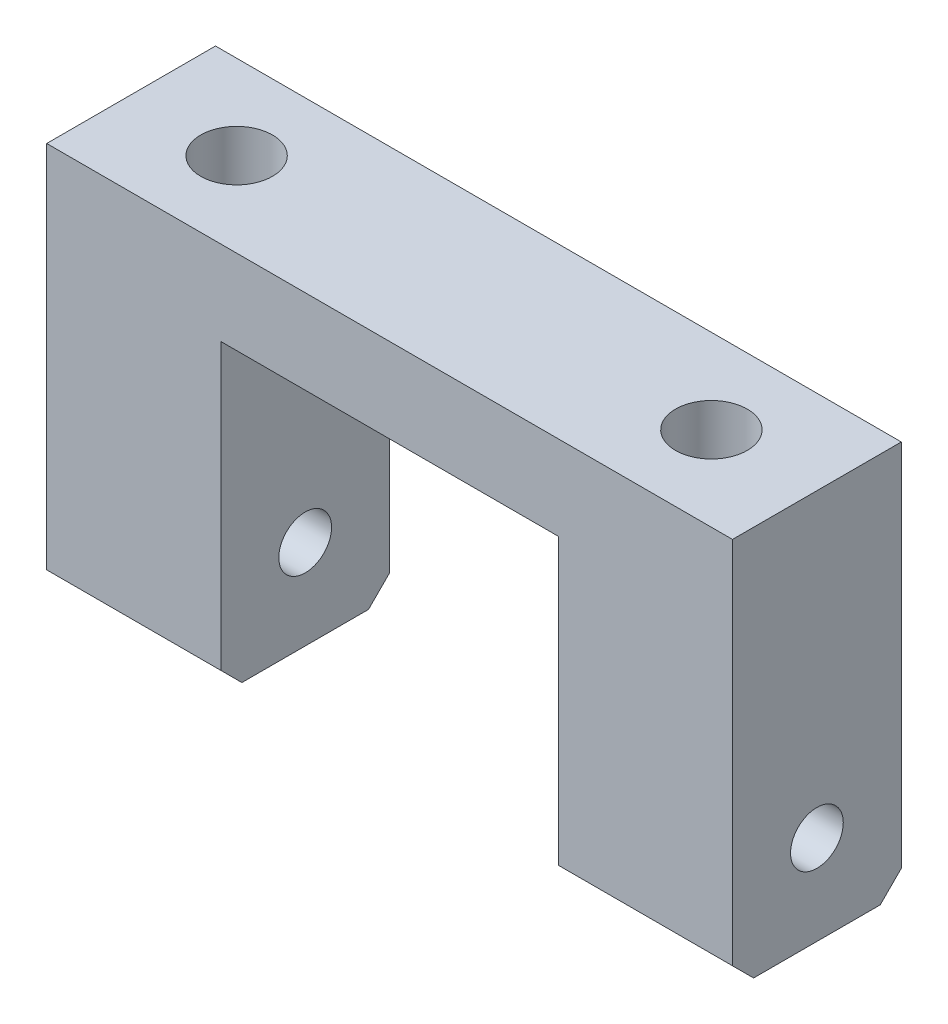
SolidWorks part; units mm, degrees
ref_plane "前视基准面" through (0, 0, 0) normal (0, 0, 1) x (1, 0, 0)
ref_plane "上视基准面" through (0, 0, 0) normal (0, 1, 0) x (1, 0, 0)
ref_plane "右视基准面" through (0, 0, 0) normal (1, 0, 0) x (0, 0, -1)
sketch "草图1" plane through (0, 0, 0) normal (0, 0, 1) x (1, 0, 0)
  line L0 (0, 18.5) -> (0, 0) construction
  line L1 (-32.5, 18.5) -> (32.5, 18.5)
  line L2 (-32.5, 18.5) -> (-32.5, -18.5)
  line L3 (-32.5, -18.5) -> (32.5, -18.5)
  line L4 (32.5, 18.5) -> (32.5, -18.5)
  line L5 (0, 0) -> (32.5, 0) construction
  dimension "D1" = 65
  dimension "D2" = 37
extrude "凸台-拉伸1" add sketch "草图1" along normal mid plane 16
sketch "草图3" plane through (0, 0, 8) normal (0, 0, 1) x (1, 0, 0)
  line L0 (-32.5, -18.5) -> (32.5, -18.5) construction
  line L1 (-16, -18.5) -> (16, -18.5)
  line L2 (-16, -18.5) -> (-16, 10.5)
  line L3 (-16, 10.5) -> (16, 10.5)
  line L4 (16, -18.5) -> (16, 10.5)
  line L5 (0, 29) -> (0, 0) construction
  line L6 (0, 0) -> (44.4811, 0) construction
  line L7 (32.5, 18.5) -> (-32.5, 18.5) construction
  dimension "D1" = 32
  dimension "D2" = 8
extrude "切除-拉伸1" cut sketch "草图3" against normal through all
hole_wizard "M6 螺纹孔1" positions "草图7" profile "草图6" tap size "M6" standard "ISO" end condition through all
sketch "草图7" plane through (32.5, 0, 0) normal (1, 0, 0) x (0, 0, -1)
  line L0 (0, 0) -> (0, -16.1416) construction
  line L4 (-8, -18.5) -> (8, -18.5) construction
  point P0 (0, -10)
  dimension "D1" = 8.5
sketch "草图6" plane through (32.5, -10, 0) normal (0, 1, 0) x (0, 0, -1)
  line L0 (0, 0) -> (0, 65)
  line L1 (0, 65) -> (2.5, 65)
  line L2 (2.5, 65) -> (2.5, 0)
  line L5 (2.5, 0) -> (0, 0)
  line L11 (0, -6.35) -> (0, 107.95) construction
  dimension "通孔螺纹孔钻头直径" = 5
  dimension "通孔螺纹孔钻头深度" = 65
cosmetic thread "孔螺蚊线4" parameters "D2"=6
hole_wizard "M8 螺纹孔1" positions "草图9" profile "草图8" tap size "M8" standard "Iso"
sketch "草图9" plane through (0, 23.5, 0) normal (0, 1, 0) x (1, 0, 0)
  line L0 (0, 13.8881) -> (0, 0) construction
  line L1 (0, 0) -> (44.4811, 0) construction
  point P0 (-32.5, 0)
  point P2 (32.5, 0)
  dimension "D1" = 65
sketch "草图8" plane through (-32.5, 23.5, 0) normal (1, 0, 0) x (0, 0, 1)
  line L0 (0, 0) -> (0, 21.7929)
  line L1 (0, 21.7929) -> (3.4, 19.75)
  line L2 (3.4, 19.75) -> (3.4, 0)
  line L5 (3.4, 0) -> (0, 0)
  line L10 (0, 21.7929) -> (-3.4, 19.75) construction
  line L11 (0, -6.35) -> (0, 107.95) construction
  dimension "螺纹孔钻头直径" = 6.8
  dimension "螺纹孔钻头深度" = 19.75
  dimension "导头角度" = 118
cosmetic thread "孔螺蚊线2" [suppressed] parameters "D1"=16, "D2"=8
cosmetic thread "孔螺蚊线3" [suppressed] parameters "D1"=16, "D2"=8
hole_wizard "M8 螺纹孔2" positions "草图11" profile "草图10" tap size "M8" standard "GB"
sketch "草图11" plane through (0, 18.5, 0) normal (0, 1, 0) x (1, 0, 0)
  line L0 (-32.5, 0) -> (32.5, 0) construction
  line L1 (-32.5, -8) -> (-32.5, 8) construction
  line L2 (32.5, -8) -> (32.5, 8) construction
  point P0 (-22.5, 0)
  point P2 (22.5, 0)
  dimension "D1" = 10
  dimension "D2" = 10
sketch "草图10" plane through (-22.5, 18.5, 0) normal (1, 0, 0) x (0, 0, 1)
  line L0 (0, 0) -> (0, 24.2929)
  line L1 (0, 24.2929) -> (3.4, 22.25)
  line L2 (3.4, 22.25) -> (3.4, 0)
  line L5 (3.4, 0) -> (0, 0)
  line L10 (0, 24.2929) -> (-3.4, 22.25) construction
  line L11 (0, -6.35) -> (0, 107.95) construction
  dimension "螺纹孔钻头直径" = 6.8
  dimension "螺纹孔钻头深度" = 22.25
  dimension "导头角度" = 118
cosmetic thread "孔螺蚊线5" parameters "D1"=16, "D2"=8
cosmetic thread "孔螺蚊线6" parameters "D1"=16, "D2"=8
chamfer "倒角1" distance 2 angle 45 4 edges at (-24.25, -18.5, -8) (-24.25, -18.5, 8) (24.25, -18.5, -8) (24.25, -18.5, 8)
